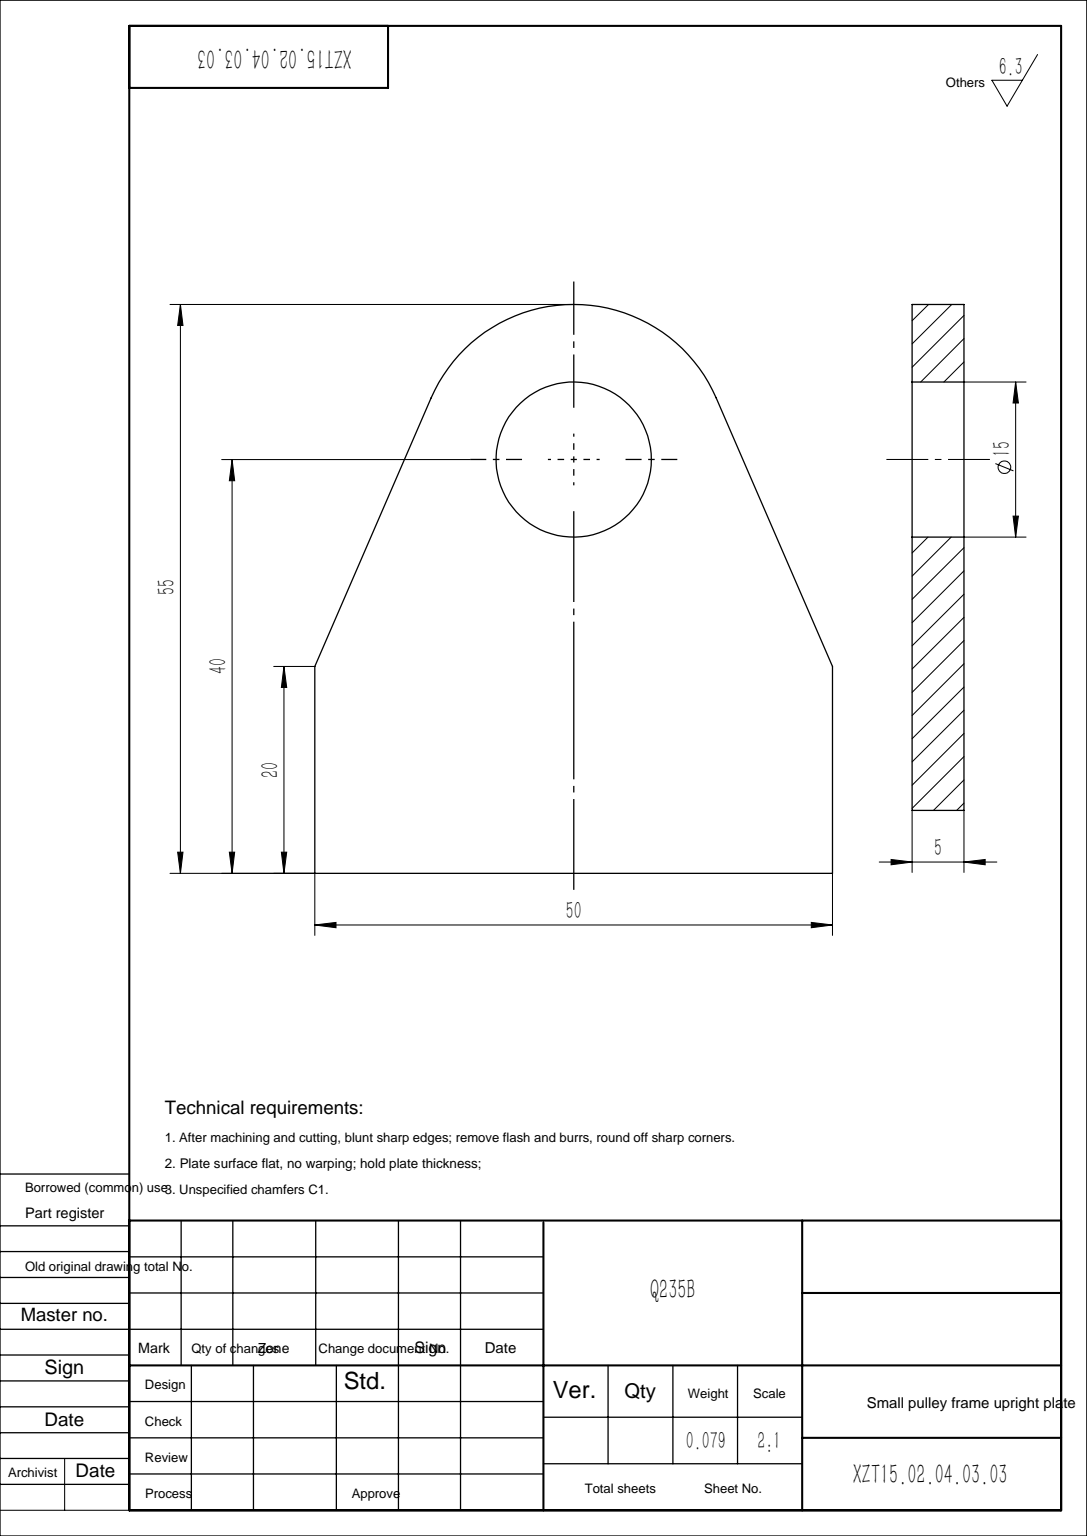
from build123d import *

# Parameters (mm, degrees)
SKETCH1_R           = 7.5
BOSS_EXTRUDE1_DEPTH = 2.5
SKETCH2_W           = 50
SKETCH2_H           = 20
BOSS_EXTRUDE2_DEPTH = 5


with BuildPart() as part:
    # Sketch1 → Boss-Extrude1 (new, symmetric)
    with BuildSketch(Plane.XY):
        with BuildLine():
            Line((25, 0), (-25, 0))
            Line((-25, 0), (-13.76612817, 25.957660212))
            ThreePointArc((-13.76612817, 25.957660212), (0, 35), (13.76612817, 25.957660212))
            Line((13.76612817, 25.957660212), (25, 0))
        make_face()
        with Locations((0, 20)):
            Circle(SKETCH1_R, mode=Mode.SUBTRACT)
    extrude(amount=BOSS_EXTRUDE1_DEPTH, both=True)

    # Sketch2 → Boss-Extrude2 (add)
    with BuildSketch(Plane.XY.offset(2.5)):
        with Locations((0, -10)):
            Rectangle(SKETCH2_W, SKETCH2_H)
    extrude(amount=-BOSS_EXTRUDE2_DEPTH)


solid = part.part
